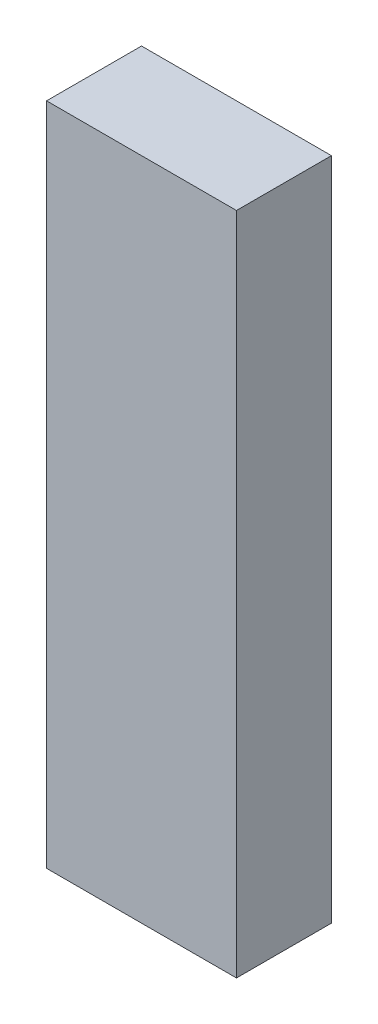
SolidWorks part; units mm, degrees
ref_plane "前视基准面" through (0, 0, 0) normal (0, 0, 1) x (1, 0, 0)
ref_plane "上视基准面" through (0, 0, 0) normal (0, 1, 0) x (1, 0, 0)
ref_plane "右视基准面" through (0, 0, 0) normal (1, 0, 0) x (0, 0, -1)
sketch "草图1" plane through (0, 0, 0) normal (0, 0, 1) x (1, 0, 0)
  line L0 (0, 0) -> (20, 0)
  line L1 (20, 0) -> (20, 70)
  line L2 (20, 70) -> (0, 70)
  line L3 (0, 70) -> (0, 0)
extrude "凸台-拉伸1" add sketch "草图1" along normal blind 10
